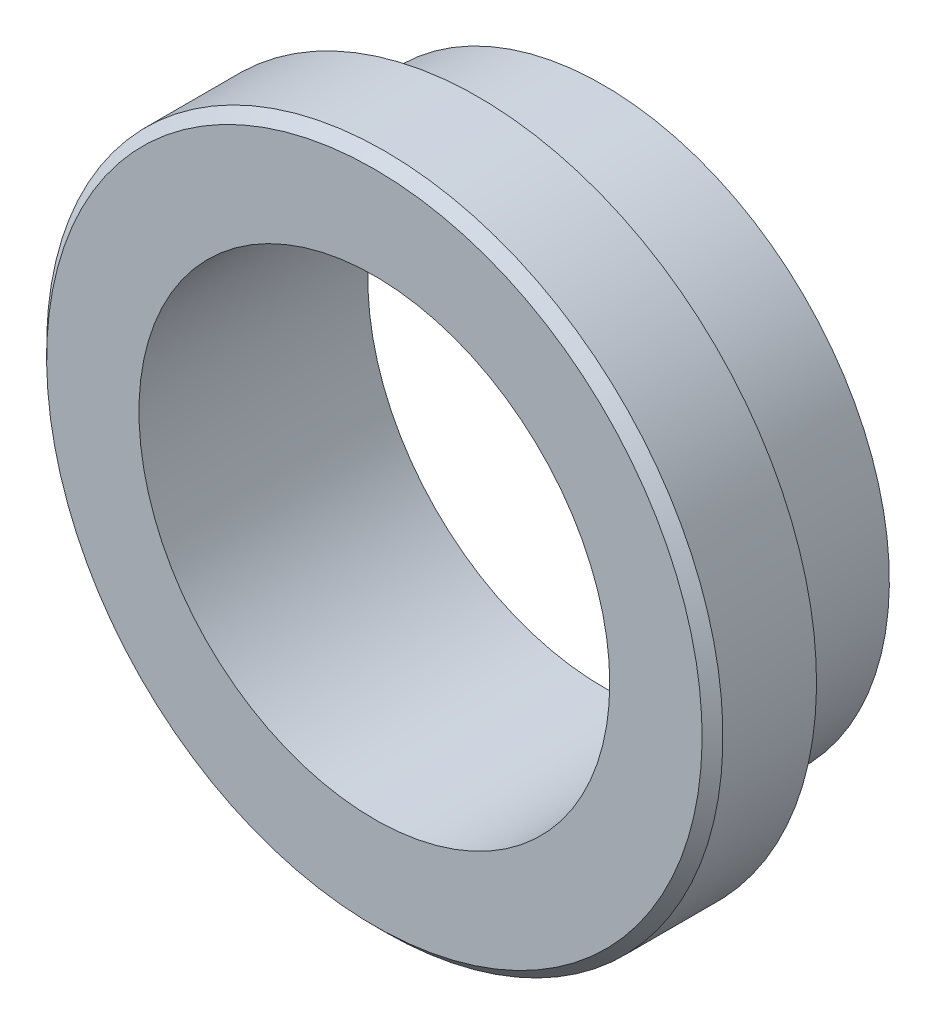
from build123d import *

# Parameters (mm, degrees)
G1_1_2_TAPPED_HOLE1_D = 45.25
CHAMFER1_SIZE         = 1


with BuildPart() as part:
    # Sketch1 → Revolve1 (revolve)
    with BuildSketch(Plane(origin=(0, 0, 0), x_dir=(0, 0, -1), z_dir=(1, 0, 0)), mode=Mode.PRIVATE) as revolve1_sk:
        Polygon((0, 0), (0, 27.5), (-12, 27.5), (-12, 32.5), (-22, 32.5), (-22, 0), align=None)
    revolve(revolve1_sk.sketch.rotate(Axis((0, 0, 22), (0, 0, -1)), 180), axis=Axis((0, 0, 22), (0, 0, -1)))

    # G1-1/2 Tapped Hole1 (through all)
    with Locations(Plane.XY.offset(22)):
        with Locations((0, 0)):
            Hole(G1_1_2_TAPPED_HOLE1_D / 2)

    # Chamfer1
    chamfer1_edges = [part.edges().sort_by_distance(p)[0] for p in [
        (0, 32.5, 22),
    ]]
    chamfer(chamfer1_edges, length=CHAMFER1_SIZE)


solid = part.part
